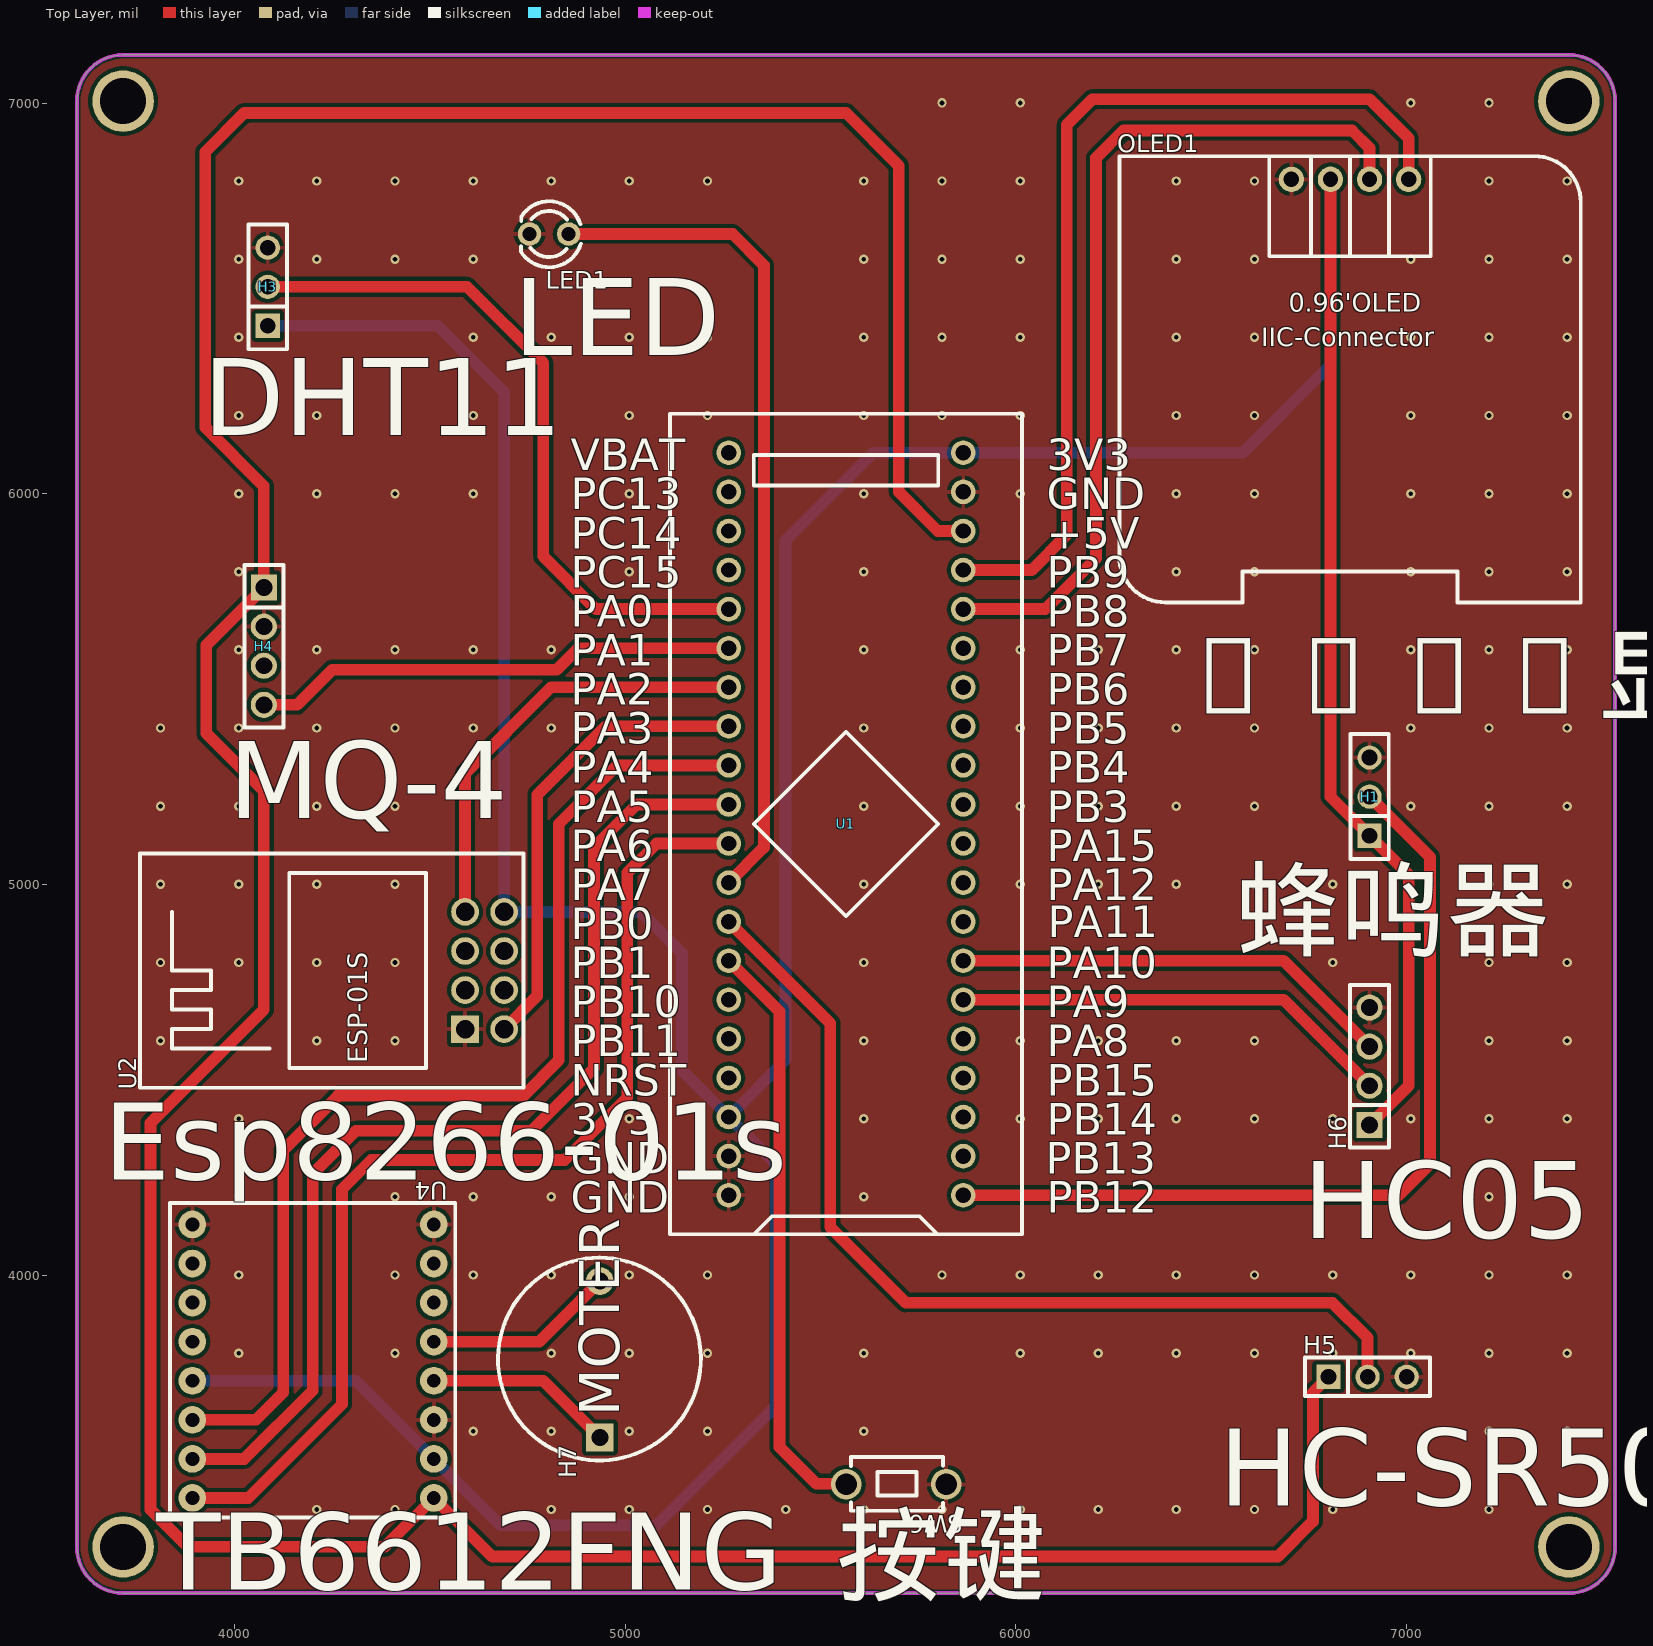
[diagram p0: Top Layer view]
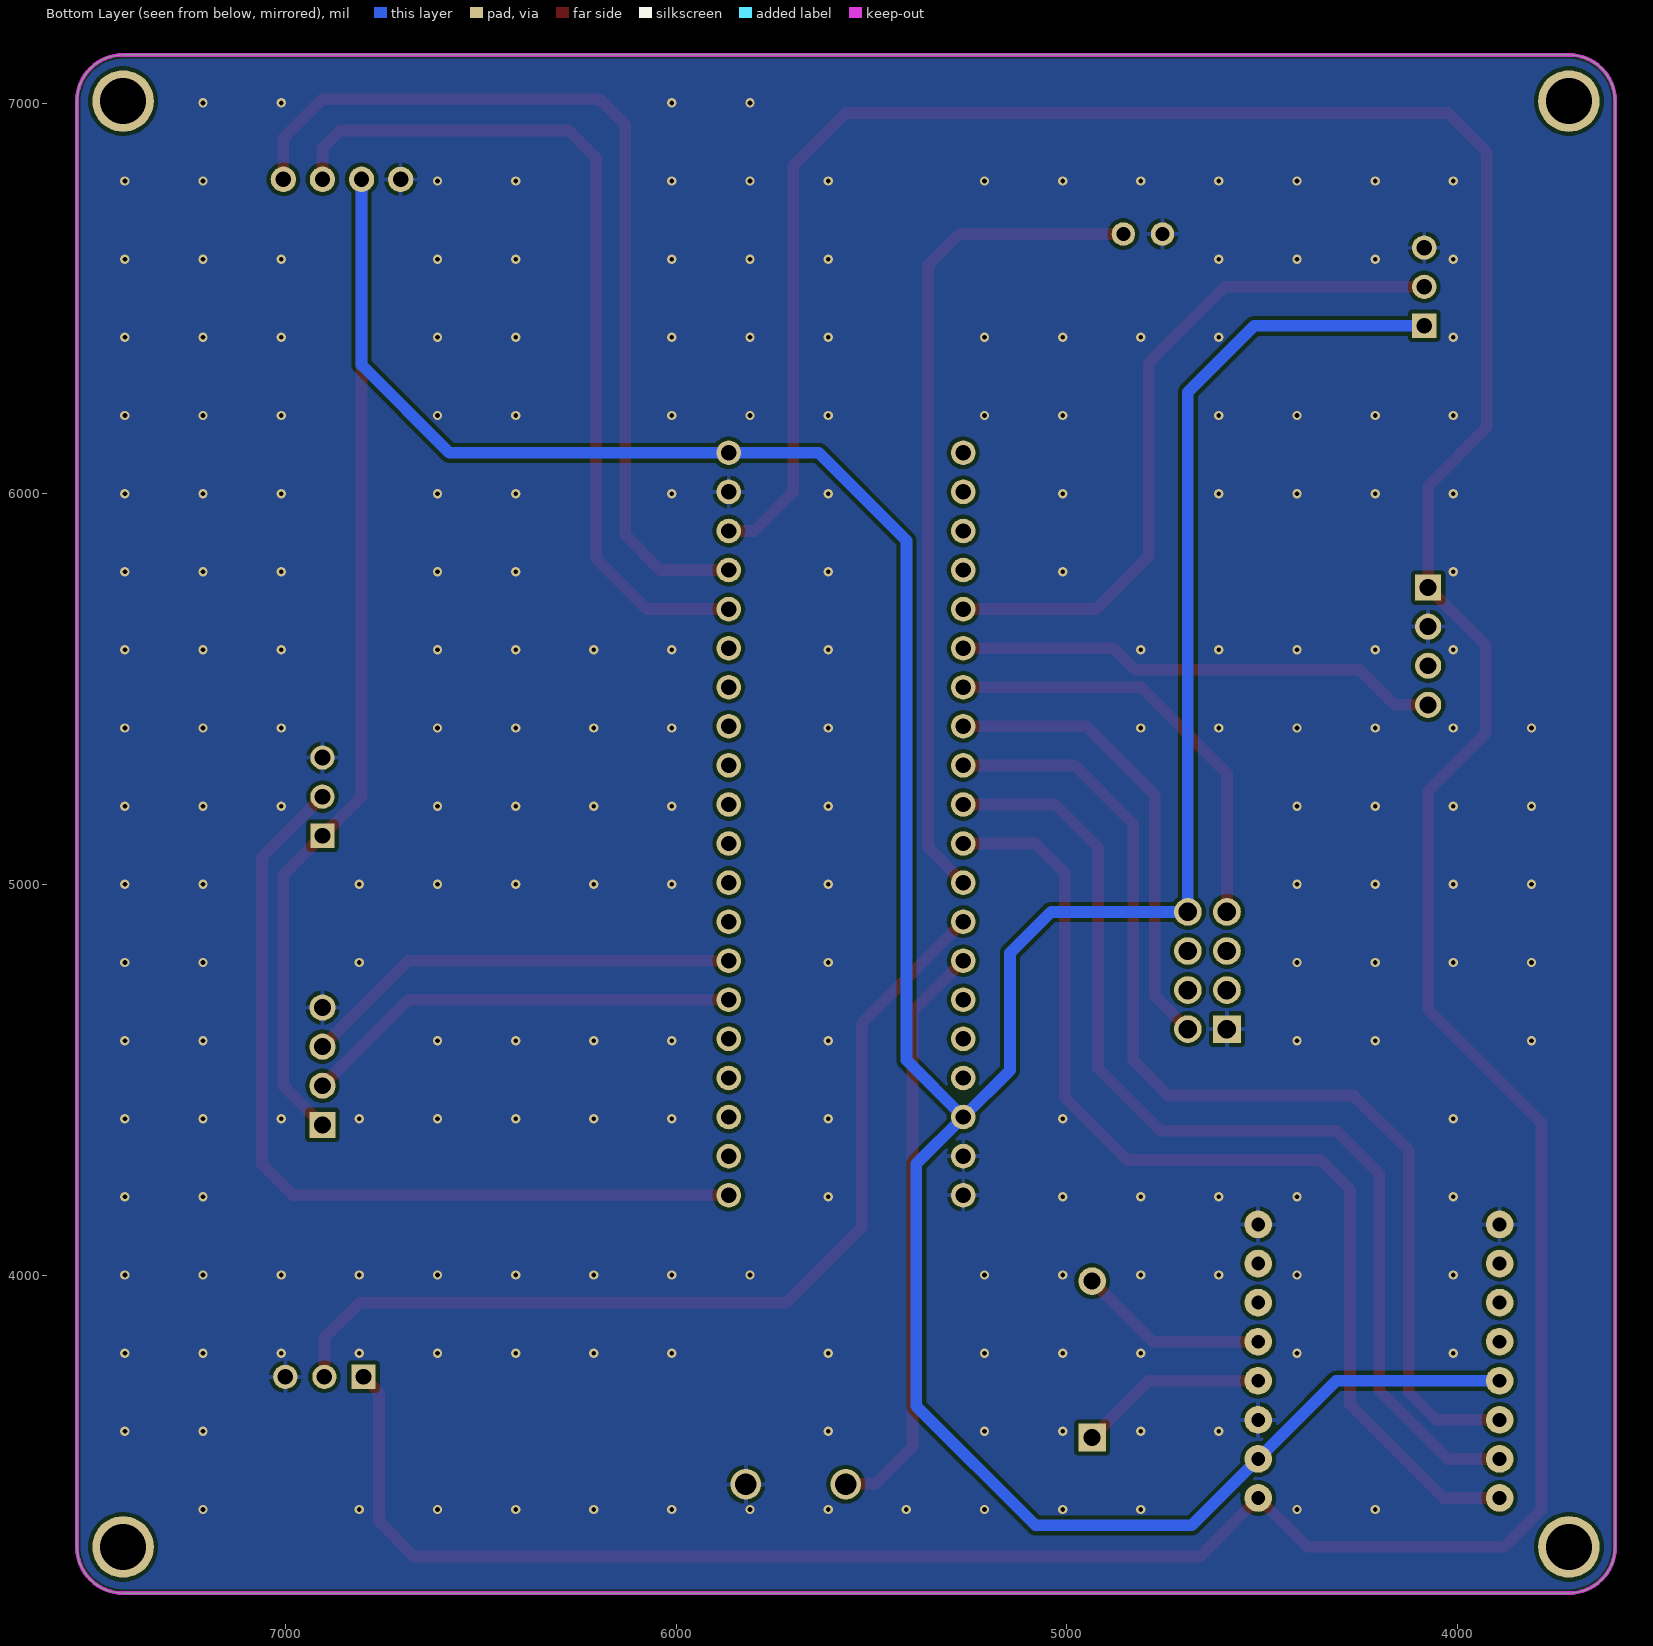
[diagram p1: Bottom Layer view, seen from below]
# Altium PCB MISC50942.pcbdoc
Units mil, origin at the board's own origin, x right, y up, seen from the top; angles counter-clockwise.
Board outline 3937.01 x 3937.01 mil, 2 copper layers (Top Layer, Bottom Layer), stack 62.206 mil thick; 12 components, 39 nets, 95 pads, 215 vias.

## Layer stack, top to bottom
Top Solder Mask Layer: solder mask 0.394, Dk 3.3
Top Layer: signal copper 1.379
Dielectric1: surface 59.449, FR4, Dk 4.5
Bottom Layer: signal copper 1.378
Bottom Solder Mask Layer: solder mask 0.394, Dk 3.3

## Board outline
3714.61,7123.5 ccw(c3714.61,7005.39) 3596.5,7005.39 3596.5,3304.61 ccw(c3714.61,3304.61) 3714.61,3186.5 7415.39,3186.5 ccw(c7415.39,3304.61) 7533.5,3304.61 7533.5,7005.39 ccw(c7415.39,7005.39) 7415.39,7123.5 3714.61,7123.5

## Design rules (kind name [scope] priority, off if disabled: settings)
BoardOutlineClearance copperThickness2oz_1 [All] p2 off: genericclearance=7.99 ignorepadtopadclearanceinfootprint=FALSE except(0: Arc-SplitContinuation Track-SplitContinuation SMDPad-SplitContinuation THPad-SplitContinuation Via-SplitContinuation Fill-SplitContinuation Region-SplitContinuation Poly-SplitContinuation Text-SplitContinuation Hole-SplitContinuation; 5.98: Arc-CutoutEdge Track-CutoutEdge SMDPad-CutoutEdge THPad-CutoutEdge Via-CutoutEdge Text-CutoutEdge; 6.9: Hole-OutlineEdge Hole-CutoutEdge; 10: Poly-OutlineEdge Poly-CutoutEdge; 11.81: Arc-OutlineEdge Track-OutlineEdge SMDPad-OutlineEdge THPad-OutlineEdge Via-OutlineEdge Fill-OutlineEdge Region-OutlineEdge Text-OutlineEdge Fill-CutoutEdge Region-CutoutEdge)
BoardOutlineClearance Plane_innerPlane_1 [All] p4 off: genericclearance=4.02 ignorepadtopadclearanceinfootprint=FALSE except(0: Arc-SplitContinuation Track-SplitContinuation SMDPad-SplitContinuation THPad-SplitContinuation Via-SplitContinuation Fill-SplitContinuation Region-SplitContinuation Poly-SplitContinuation Text-SplitContinuation Hole-SplitContinuation; 5.98: Arc-CutoutEdge Track-CutoutEdge SMDPad-CutoutEdge THPad-CutoutEdge Via-CutoutEdge Text-CutoutEdge; 6.9: Hole-OutlineEdge Hole-CutoutEdge; 10: Poly-OutlineEdge Poly-CutoutEdge; 11.81: Arc-OutlineEdge Track-OutlineEdge SMDPad-OutlineEdge THPad-OutlineEdge Via-OutlineEdge Fill-OutlineEdge Region-OutlineEdge Text-OutlineEdge Fill-CutoutEdge Region-CutoutEdge)
BoardOutlineClearance Copper_copperRegion_1 [All] p6 off: genericclearance=4.02 ignorepadtopadclearanceinfootprint=FALSE except(0: Arc-SplitContinuation Track-SplitContinuation SMDPad-SplitContinuation THPad-SplitContinuation Via-SplitContinuation Fill-SplitContinuation Region-SplitContinuation Poly-SplitContinuation Text-SplitContinuation Hole-SplitContinuation; 5.98: Arc-CutoutEdge Track-CutoutEdge SMDPad-CutoutEdge THPad-CutoutEdge Via-CutoutEdge Text-CutoutEdge; 6.9: Hole-OutlineEdge Hole-CutoutEdge; 10: Poly-OutlineEdge Poly-CutoutEdge; 11.81: Arc-OutlineEdge Track-OutlineEdge SMDPad-OutlineEdge THPad-OutlineEdge Via-OutlineEdge Fill-OutlineEdge Region-OutlineEdge Text-OutlineEdge Fill-CutoutEdge Region-CutoutEdge)
BoardOutlineClearance Copper_copperRegion_copperThickness1oz_1 [All] p8 off: genericclearance=4.02 ignorepadtopadclearanceinfootprint=FALSE except(0: Arc-SplitContinuation Track-SplitContinuation SMDPad-SplitContinuation THPad-SplitContinuation Via-SplitContinuation Fill-SplitContinuation Region-SplitContinuation Poly-SplitContinuation Text-SplitContinuation Hole-SplitContinuation; 5.98: Arc-CutoutEdge Track-CutoutEdge SMDPad-CutoutEdge THPad-CutoutEdge Via-CutoutEdge Text-CutoutEdge; 6.9: Hole-OutlineEdge Hole-CutoutEdge; 10: Poly-OutlineEdge Poly-CutoutEdge; 11.81: Arc-OutlineEdge Track-OutlineEdge SMDPad-OutlineEdge THPad-OutlineEdge Via-OutlineEdge Fill-OutlineEdge Region-OutlineEdge Text-OutlineEdge Fill-CutoutEdge Region-CutoutEdge)
BoardOutlineClearance Copper_copperRegion_Copper_copperRegion_1 [All] p10 off: genericclearance=4.02 ignorepadtopadclearanceinfootprint=FALSE except(0: Arc-SplitContinuation Track-SplitContinuation SMDPad-SplitContinuation THPad-SplitContinuation Via-SplitContinuation Fill-SplitContinuation Region-SplitContinuation Poly-SplitContinuation Text-SplitContinuation Hole-SplitContinuation; 5.98: Arc-CutoutEdge Track-CutoutEdge SMDPad-CutoutEdge THPad-CutoutEdge Via-CutoutEdge Text-CutoutEdge; 6.9: Hole-OutlineEdge Hole-CutoutEdge; 10: Poly-OutlineEdge Poly-CutoutEdge; 11.81: Arc-OutlineEdge Track-OutlineEdge SMDPad-OutlineEdge THPad-OutlineEdge Via-OutlineEdge Fill-OutlineEdge Region-OutlineEdge Text-OutlineEdge Fill-CutoutEdge Region-CutoutEdge)
BoardOutlineClearance copperThickness1oz_1 [All] p12: genericclearance=4.02 ignorepadtopadclearanceinfootprint=FALSE except(0: Arc-SplitContinuation Track-SplitContinuation SMDPad-SplitContinuation THPad-SplitContinuation Via-SplitContinuation Fill-SplitContinuation Region-SplitContinuation Poly-SplitContinuation Text-SplitContinuation Hole-SplitContinuation; 5.98: Arc-CutoutEdge Track-CutoutEdge SMDPad-CutoutEdge THPad-CutoutEdge Via-CutoutEdge Text-CutoutEdge; 6.9: Hole-OutlineEdge Hole-CutoutEdge; 10: Poly-OutlineEdge Poly-CutoutEdge; 11.81: Arc-OutlineEdge Track-OutlineEdge SMDPad-OutlineEdge THPad-OutlineEdge Via-OutlineEdge Fill-OutlineEdge Region-OutlineEdge Text-OutlineEdge Fill-CutoutEdge Region-CutoutEdge)
Clearance copperThickness2oz [All] p1 off: gap=7.99 ignorepadtopadclearanceinfootprint=FALSE except(5.98: SMDPad-Track SMDPad-SMDPad THPad-Track SMDPad-THPad THPad-THPad Track-Via SMDPad-Via THPad-Via Via-Via Fill-SMDPad Region-SMDPad Fill-THPad Region-THPad Fill-Via Region-Via Fill-Fill Fill-Region Region-Region Arc-Track Arc-SMDPad Arc-THPad Arc-Via Fill-Arc Region-Arc Arc-Arc Text-Track SMDPad-Text Text-THPad Text-Via Fill-Text Region-Text Arc-Text Text-Text; 6.9: Hole-Track Hole-SMDPad Hole-THPad Hole-Via Fill-Hole Region-Hole Hole-Arc Hole-Text; 10: Poly-Track Poly-SMDPad Poly-THPad Poly-Via Poly-Fill Poly-Region Poly-Poly Poly-Arc Poly-Text Poly-Hole; 11.81: Fill-Track Region-Track)
Clearance Plane_innerPlane [All] p3 off: gap=4.02 ignorepadtopadclearanceinfootprint=FALSE except(5.98: SMDPad-Track SMDPad-SMDPad THPad-Track SMDPad-THPad THPad-THPad Track-Via SMDPad-Via THPad-Via Via-Via Fill-SMDPad Region-SMDPad Fill-THPad Region-THPad Fill-Via Region-Via Fill-Fill Fill-Region Region-Region Arc-Track Arc-SMDPad Arc-THPad Arc-Via Fill-Arc Region-Arc Arc-Arc Text-Track SMDPad-Text Text-THPad Text-Via Fill-Text Region-Text Arc-Text Text-Text; 6.9: Hole-Track Hole-SMDPad Hole-THPad Hole-Via Fill-Hole Region-Hole Hole-Arc Hole-Text; 10: Poly-Track Poly-SMDPad Poly-THPad Poly-Via Poly-Fill Poly-Region Poly-Poly Poly-Arc Poly-Text Poly-Hole; 11.81: Fill-Track Region-Track)
Clearance Copper_copperRegion [All] p5 off: gap=4.02 ignorepadtopadclearanceinfootprint=FALSE except(5.98: SMDPad-Track SMDPad-SMDPad THPad-Track SMDPad-THPad THPad-THPad Track-Via SMDPad-Via THPad-Via Via-Via Fill-SMDPad Region-SMDPad Fill-THPad Region-THPad Fill-Via Region-Via Fill-Fill Fill-Region Region-Region Arc-Track Arc-SMDPad Arc-THPad Arc-Via Fill-Arc Region-Arc Arc-Arc Text-Track SMDPad-Text Text-THPad Text-Via Fill-Text Region-Text Arc-Text Text-Text; 6.9: Hole-Track Hole-SMDPad Hole-THPad Hole-Via Fill-Hole Region-Hole Hole-Arc Hole-Text; 10: Poly-Track Poly-SMDPad Poly-THPad Poly-Via Poly-Fill Poly-Region Poly-Poly Poly-Arc Poly-Text Poly-Hole; 11.81: Fill-Track Region-Track)
Clearance Copper_copperRegion_copperThickness1oz [All] p7 off: gap=4.02 ignorepadtopadclearanceinfootprint=FALSE except(5.98: SMDPad-Track SMDPad-SMDPad THPad-Track SMDPad-THPad THPad-THPad Track-Via SMDPad-Via THPad-Via Via-Via Fill-SMDPad Region-SMDPad Fill-THPad Region-THPad Fill-Via Region-Via Fill-Fill Fill-Region Region-Region Arc-Track Arc-SMDPad Arc-THPad Arc-Via Fill-Arc Region-Arc Arc-Arc Text-Track SMDPad-Text Text-THPad Text-Via Fill-Text Region-Text Arc-Text Text-Text; 6.9: Hole-Track Hole-SMDPad Hole-THPad Hole-Via Fill-Hole Region-Hole Hole-Arc Hole-Text; 10: Poly-Track Poly-SMDPad Poly-THPad Poly-Via Poly-Fill Poly-Region Poly-Poly Poly-Arc Poly-Text Poly-Hole; 11.81: Fill-Track Region-Track)
Clearance Copper_copperRegion_Copper_copperRegion [All] p9 off: gap=4.02 ignorepadtopadclearanceinfootprint=FALSE except(5.98: SMDPad-Track SMDPad-SMDPad THPad-Track SMDPad-THPad THPad-THPad Track-Via SMDPad-Via THPad-Via Via-Via Fill-SMDPad Region-SMDPad Fill-THPad Region-THPad Fill-Via Region-Via Fill-Fill Fill-Region Region-Region Arc-Track Arc-SMDPad Arc-THPad Arc-Via Fill-Arc Region-Arc Arc-Arc Text-Track SMDPad-Text Text-THPad Text-Via Fill-Text Region-Text Arc-Text Text-Text; 6.9: Hole-Track Hole-SMDPad Hole-THPad Hole-Via Fill-Hole Region-Hole Hole-Arc Hole-Text; 10: Poly-Track Poly-SMDPad Poly-THPad Poly-Via Poly-Fill Poly-Region Poly-Poly Poly-Arc Poly-Text Poly-Hole; 11.81: Fill-Track Region-Track)
Clearance copperThickness1oz [All] p11: gap=4.02 ignorepadtopadclearanceinfootprint=FALSE except(5.98: SMDPad-Track SMDPad-SMDPad THPad-Track SMDPad-THPad THPad-THPad Track-Via SMDPad-Via THPad-Via Via-Via Fill-SMDPad Region-SMDPad Fill-THPad Region-THPad Fill-Via Region-Via Fill-Fill Fill-Region Region-Region Arc-Track Arc-SMDPad Arc-THPad Arc-Via Fill-Arc Region-Arc Arc-Arc Text-Track SMDPad-Text Text-THPad Text-Via Fill-Text Region-Text Arc-Text Text-Text; 6.9: Hole-Track Hole-SMDPad Hole-THPad Hole-Via Fill-Hole Region-Hole Hole-Arc Hole-Text; 10: Poly-Track Poly-SMDPad Poly-THPad Poly-Via Poly-Fill Poly-Region Poly-Poly Poly-Arc Poly-Text Poly-Hole; 11.81: Fill-Track Region-Track)
DiffPairsRouting differentialPair [All] p1: maxlimit=6 minlimit=6 mostfreqgap=6 toplayer_minwidth=5 toplayer_prefwidth=10 toplayer_maxwidth=100 toplayer_mingap=6 toplayer_prefgap=6 toplayer_maxgap=6 bottomlayer_minwidth=5 bottomlayer_prefwidth=10 bottomlayer_maxwidth=100 bottomlayer_mingap=6 bottomlayer_prefgap=6 bottomlayer_maxgap=6 maxuncoupledlength=10
HoleToHoleClearance otherClearance [All] p1: gap=11.81 allowstackedmicrovias=TRUE
Length netLength [All] p1: minlimit=0 maxlimit=0
PasteMaskExpansion pasteMaskExpansion [All] p1: expansion=0
PlaneConnect innerPlane [All] p1: planeconnectstyle=Relief reliefexpansion=20 reliefentries=4 reliefconductorwidth=10 reliefairgap=10
PolygonConnect copperRegion_copperThickness1oz [All] p1 off: connectstyle=Relief reliefconductorwidth=10 reliefentries=4 polygonreliefangle="90 Angle" airgapwidth=10 via.connectstyle=Relief via.reliefconductorwidth=10 via.reliefentries=4 via.polygonreliefangle="90 Angle" via.airgapwidth=10
PolygonConnect copperRegion_Copper_copperRegion [All] p2 off: connectstyle=Relief reliefconductorwidth=10 reliefentries=4 polygonreliefangle="90 Angle" airgapwidth=10 via.connectstyle=Relief via.reliefconductorwidth=10 via.reliefentries=4 via.polygonreliefangle="90 Angle" via.airgapwidth=10
PolygonConnect copperRegion [All] p3: connectstyle=Relief reliefconductorwidth=10 reliefentries=4 polygonreliefangle="90 Angle" airgapwidth=10 via.connectstyle=Relief via.reliefconductorwidth=10 via.reliefentries=4 via.polygonreliefangle="90 Angle" via.airgapwidth=10
RoutingVias viaSize [All] p1: holewidth=12.01 width=24.02 viastyle="Through Hole" minholewidth=11.81 minwidth=19.68 maxholewidth=248.03 maxwidth=393.7
SolderMaskExpansion solderMaskExpansion [IsVia] p1: expansion=-1000 istentingtop=TRUE
SolderMaskExpansion solderMaskExpansion [All] p2: expansion=2 istentingtop=FALSE
Width copperThickness2oz_2 [All] p1 off: maxlimit=100 minlimit=8 preferedwidth=10
Width copperThickness1oz_2 [All] p2: maxlimit=100 minlimit=5 preferedwidth=10

## Components (designator, comment, footprint, x,y, rotation, side; value= is the part's Value field where it differs from the comment)
H1 "" HDR-TH_3P-P2.54-V-F 6905,5225 r90 top
H3 "" HDR-TH_3P-P2.54-V-F 4085,6530 r90 top
H4 "" HDR-TH_4P-P2.54-V-F 4075,5610 r270 top
H5 "" HDR-TH_3P-P2.54-V-F 6900,3740 r0 top
H6 "" HDR-TH_4P-P2.54-V-F 6905,4535 r90 top
H7 "" HDR-TH_2P-P2.54-V-M-1 4935,3585 r90 top
LED1 "" LED_TH-3mm 4805,6665 r180 top
OLED1 "" 0.96OLED_4P 6855,6805 r0 top
SW6 "" Key_TH_3.5x6x4.3 5700,3465 r180 top
U1 "STM32F103C8T6-Card" CONN-TH_L53.3-W22.9_STM32F103C8T6-CARD 5565,5155 r90 top
U2 "ESP-01S" WIFIM-TH_ESP-01S 4640,4780 r90 top
U4 "" tb6612 4510,3430 r180 top

## Footprints (in the part's own frame and the unit in brackets; to place one, negate y for a bottom-side part, rotate by r counter-clockwise, add the part's x,y. Pads: shape width x height; smd on the part's side, far side on the other; paste and mask are expansions set on the pad)
0.96OLED_4P [mm]
  round 1.65 hole 1 copper offset 0,0: 1(-3.81,-0.001) 2(-1.27,0.002) 3(1.27,0.002) 4(3.81,0.002)
  silkscreen extent -15,-27.5 15,1.5
CONN-TH_L53.3-W22.9_STM32F103C8T6-CARD [mm]
  round 1.6 hole 1: 1(-24.13,-7.62) 2(-21.59,-7.62) 3(-19.05,-7.62) 4(-16.51,-7.62) 5(-13.97,-7.62) 6(-11.43,-7.62) 7(-8.89,-7.62) 8(-6.35,-7.62) 9(-3.81,-7.62) 10(-1.27,-7.62) 11(1.27,-7.62) 12(3.81,-7.62) 13(6.35,-7.62) 14(8.89,-7.62) 15(11.43,-7.62) 16(13.97,-7.62) 17(16.51,-7.62) 18(19.05,-7.62) 19(21.59,-7.62) 20(24.13,-7.62) 21(24.13,7.62) 22(21.59,7.62) 23(19.05,7.62) 24(16.51,7.62) 25(13.97,7.62) 26(11.43,7.62) 27(8.89,7.62) 28(6.35,7.62) 29(3.81,7.62) 30(1.27,7.62) 31(-1.27,7.62) 32(-3.81,7.62) 33(-6.35,7.62) 34(-8.89,7.62) 35(-11.43,7.62) 36(-13.97,7.62) 37(-16.51,7.62) 38(-19.05,7.62) 39(-21.59,7.62) 40(-24.13,7.62)
  silkscreen extent -26.67,-11.43 26.67,11.43
HDR-TH_2P-P2.54-V-M-1 [mm]
  rect 1.8x1.8 hole 1.1: 1(0,0)
  round 1.8 hole 1.1: 2(10.16,0)
  silkscreen extent -1.49,-6.56 11.69,6.62
HDR-TH_3P-P2.54-V-F [mil]
  rect 62x62 hole 40.16: 1(-100,0)
  round 62 hole 40.16: 2(0,0) 3(100,0)
  silkscreen extent -160,-49 160,49
HDR-TH_4P-P2.54-V-F [mm]
  rect 1.7x1.7 hole 1.1: 1(-3.81,0)
  round 1.7 hole 1.1: 2(-1.27,0) 3(1.27,0) 4(3.81,0)
  silkscreen extent -5.29,-1.27 5.29,1.27
Key_TH_3.5x6x4.3 [mil]
  round 78.7 hole 55.1 paste+0 mask+2: A(-121.44,0) B(134.46,0)
  silkscreen extent -114,-70 123,68
LED_TH-3mm [mil]
  round 60 hole 36 paste+0 mask+2: 1(-50,0) 2(50,0)
  silkscreen extent -81,-84 72,85
tb6612 [mm]
  round 1.8 hole 0.9: 1(0,0) 2(0,-2.54) 3(0,-5.08) 4(0,-7.62) 5(0,-10.16) 6(0,-12.7) 7(0,-15.24) 8(0,-17.78) 9(15.697,-17.78) 10(15.697,-15.24) 11(15.697,-12.7) 12(15.697,-10.16) 13(15.697,-7.62) 14(15.697,-5.08) 15(15.697,-2.54) 16(15.697,0)
  silkscreen extent -1.4,-19.18 17.15,1.27
WIFIM-TH_ESP-01S [mm]
  rect 1.8x1.8 hole 1.2: 1(-3.81,1.27)
  round 1.8 hole 1.2: 2(-1.27,1.27) 3(1.27,1.27) 4(3.81,1.27) 5(3.81,-1.27) 6(1.27,-1.27) 7(-1.27,-1.27) 8(-3.81,-1.27)
  silkscreen extent -7.62,-2.54 7.62,22.4

## Free pads (board coordinates)
  round 157.48 hole 118.11: 1(3714.61,7005.39) 1(3714.61,3304.61) 1(7415.39,7005.39) 1(7415.39,3304.61)

## Via types
v1: diameter 24.02, hole 12, Top Layer to Bottom Layer, 215 vias

## Nets (pads, with @x,y where several pads share a name; then routed paths per layer and width w, separated by ;. In a path a pad name is that pad's centre, name@x,y a point inside that pad or via, vN(x,y) a via of type N, cw(c..) or ccw(c..) an arc to the next point about the centre after c; other vN are vias at no path point)
$1N17162: H7.1 U4.4 | length 485.1
  Top Layer w30: U4.4 4790,3730 H7.1
$1N17163: H7.2 U4.5 | length 489.2
  Top Layer w30: U4.5 4780,3830 H7.2
+5V: H4.1 H5.1 U1.18 U4.1 | length 10245
  Top Layer w30: U1.18 5800,5905 5700,6005 5700,6840 5565,6975 4025,6975 3925,6875 3925,6170 4075,6020 H4.1 3927.93,5612.93 3927.93,5387.07 4075,5240 4075,4680 3785,4390 3785,3400 3880,3305 4385,3305 U4.1 4660,3280 6670,3280 6760,3370 6760,3700 H5.1
GND: H1.3 H3.3 H4.2 H5.3 H6.4 LED1.2 OLED1.1 SW6.A U1.19 U1.39 U1.40 U2.1 U4.3 U4.8 U4.9
  other v1: 4210.6,3400.6 4410.6,3400.6 4810.6,3400.6 5010.6,3400.6 5210.6,3400.6 5410.6,3400.6 5610.6,3400.6 5810.6,3400.6 6010.6,3400.6 6210.6,3400.6 6410.6,3400.6 6610.6,3400.6 6810.6,3400.6 7210.6,3400.6 4610.6,3600.6 4810.6,3600.6 5010.6,3600.6 5210.6,3600.6 5610.6,3600.6 7210.6,3600.6 7410.6,3600.6 4010.6,3800.6 4410.6,3800.6 4810.6,3800.6 5010.6,3800.6 5210.6,3800.6 5610.6,3800.6 6010.6,3800.6 6210.6,3800.6 6410.6,3800.6 6610.6,3800.6 6810.6,3800.6 7010.6,3800.6 7210.6,3800.6 7410.6,3800.6 4010.6,4000.6 4410.6,4000.6 4610.6,4000.6 4810.6,4000.6 5010.6,4000.6 5210.6,4000.6 5810.6,4000.6 6010.6,4000.6 6210.6,4000.6 6410.6,4000.6 6610.6,4000.6 6810.6,4000.6 7010.6,4000.6 7210.6,4000.6 7410.6,4000.6 4010.6,4200.6 4410.6,4200.6 4610.6,4200.6 4810.6,4200.6 5010.6,4200.6 5610.6,4200.6 7210.6,4200.6 7410.6,4200.6 4010.6,4400.6 5010.6,4400.6 5610.6,4400.6 6010.6,4400.6 6210.6,4400.6 6410.6,4400.6 6610.6,4400.6 6810.6,4400.6 7010.6,4400.6 7210.6,4400.6 7410.6,4400.6 3810.6,4600.6 4210.6,4600.6 4410.6,4600.6 5610.6,4600.6 6010.6,4600.6 6210.6,4600.6 6410.6,4600.6 6610.6,4600.6 7210.6,4600.6 7410.6,4600.6 3810.6,4800.6 4010.6,4800.6 4210.6,4800.6 4410.6,4800.6 5610.6,4800.6 6810.6,4800.6 7210.6,4800.6 7410.6,4800.6 3810.6,5000.6 4010.6,5000.6 4210.6,5000.6 4410.6,5000.6 5610.6,5000.6 6010.6,5000.6 6210.6,5000.6 6410.6,5000.6 6610.6,5000.6 6810.6,5000.6 7210.6,5000.6 7410.6,5000.6 3810.6,5200.6 4010.6,5200.6 4210.6,5200.6 4410.6,5200.6 5610.6,5200.6 6010.6,5200.6 6210.6,5200.6 6410.6,5200.6 6610.6,5200.6 7010.6,5200.6 7210.6,5200.6 7410.6,5200.6 3810.6,5400.6 4010.6,5400.6 4210.6,5400.6 4410.6,5400.6 4610.6,5400.6 4810.6,5400.6 5610.6,5400.6 6010.6,5400.6 6210.6,5400.6 6410.6,5400.6 6610.6,5400.6 7010.6,5400.6 7210.6,5400.6 7410.6,5400.6 4010.6,5600.6 4210.6,5600.6 4410.6,5600.6 4610.6,5600.6 4810.6,5600.6 5610.6,5600.6 6010.6,5600.6 6210.6,5600.6 6410.6,5600.6 6610.6,5600.6 7010.6,5600.6 7210.6,5600.6 7410.6,5600.6 4010.6,5800.6 5010.6,5800.6 5610.6,5800.6 6410.6,5800.6 6610.6,5800.6 7010.6,5800.6 7210.6,5800.6 7410.6,5800.6 4010.6,6000.6 4210.6,6000.6 4410.6,6000.6 4610.6,6000.6 5010.6,6000.6 5610.6,6000.6 6010.6,6000.6 6410.6,6000.6 6610.6,6000.6 7010.6,6000.6 7210.6,6000.6 7410.6,6000.6 4010.6,6200.6 4210.6,6200.6 4410.6,6200.6 4610.6,6200.6 5010.6,6200.6 5210.6,6200.6 5610.6,6200.6 5810.6,6200.6 6010.6,6200.6 6410.6,6200.6 6610.6,6200.6 7010.6,6200.6 7210.6,6200.6 7410.6,6200.6 4010.6,6400.6 4610.6,6400.6 4810.6,6400.6 5010.6,6400.6 5210.6,6400.6 5610.6,6400.6 5810.6,6400.6 6010.6,6400.6 6410.6,6400.6 6610.6,6400.6 7010.6,6400.6 7210.6,6400.6 7410.6,6400.6 4010.6,6600.6 4210.6,6600.6 4410.6,6600.6 4610.6,6600.6 5610.6,6600.6 5810.6,6600.6 6010.6,6600.6 6410.6,6600.6 6610.6,6600.6 7010.6,6600.6 7210.6,6600.6 7410.6,6600.6 4010.6,6800.6 4210.6,6800.6 4410.6,6800.6 4610.6,6800.6 4810.6,6800.6 5010.6,6800.6 5210.6,6800.6 5610.6,6800.6 5810.6,6800.6 6010.6,6800.6 6410.6,6800.6 6610.6,6800.6 7210.6,6800.6 7410.6,6800.6 5810.6,7000.6 6010.6,7000.6 7010.6,7000.6 7210.6,7000.6
NRST: U1.37
PA0: H3.2 U1.25 | length 1811.7
  Top Layer w30: H3.2 4595,6530 4790,6335 4790,5840 4925,5705 U1.25
PA1: H4.4 U1.26 | length 1250.1
  Top Layer w30: H4.4 4160,5460 4250,5550 4825,5550 4880,5605 U1.26
PA2: U1.27 U2.4 | length 1121.1
  Top Layer w30: U2.4 4590,5285 4810,5505 U1.27
PA3: U1.28 U2.8 | length 1197.7
  Top Layer w30: U2.8 4775,4715 4775,5230 4950,5405 U1.28
PA4: U1.29 U4.14 | length 2784.4
  Top Layer w30: U4.14 4055,3630 4125,3700 4125,4320 4265,4460 4740,4460 4830,4550 4830,5155 4980,5305 U1.29
PA5: U1.30 U4.15 | length 2722.9
  Top Layer w30: U4.15 4025,3530 4200,3705 4200,4260 4310,4370 4760,4370 4920,4530 4920,5095 5030,5205 U1.30
PA6: U1.31 U4.16 | length 2725.8
  Top Layer w30: U4.16 4035,3430 4275,3670 4275,4220 4350,4295 4845,4295 5005,4455 5005,5030 5080,5105 U1.31
PA7: LED1.1 U1.32 | length 2150.4
  Top Layer w30: LED1.1 5275,6665 5355,6585 5355,5095 U1.32
PA8: U1.5
PA9: H6.2 U1.6 | length 1131.1
  Top Layer w30: U1.6 6685,4705 H6.2
PA10: H6.3 U1.7 | length 1131.1
  Top Layer w30: U1.7 6685,4805 H6.3
PA11: U1.8
PA12: U1.9
PA15: U1.10
PB0: H5.2 U1.33 | length 2481.8
  Top Layer w30: U1.33 5525,4645 5525,4123.27 5718.27,3930 6810,3930 6900,3840 H5.2
PB1: SW6.B U1.34 | length 1504.7
  Top Layer w30: U1.34 5395,4675 5395,3560 5488.58,3466.42 SW6.B@5562.05,3466.42
PB3: U1.11
PB4: U1.12
PB5: U1.13
PB6: U1.14
PB7: U1.15
PB8: OLED1.3 U1.16 | length 2246.4
  Top Layer w30: U1.16 6075,5705 6205,5835 6205,6860 6275,6930 6860,6930 6905,6885 OLED1.3@6905,6805.05
PB9: OLED1.4 U1.17 | length 2400.6
  Top Layer w30: U1.17 6040,5805 6130,5895 6130,6945 6195,7010 6905,7010 7005,6910 OLED1.4@7005,6805.05
PB10: U1.35
PB11: U1.36
PB12: H1.2 U1.1 | length 2232.3
  Top Layer w30: U1.1 6980,4205 7060,4285 7060,5070 H1.2
PB13: U1.2
PB14: U1.3
PB15: U1.4
PC13: U1.22
PC14: U1.23
PC15: U1.24
VBAT: U1.21
VCC: H1.1 H3.1 H6.1 OLED1.2 U1.20 U1.38 U2.5 U4.2 U4.13 | length 11671.7
  Top Layer w30: OLED1.2@6805,6805.05 6805,5225 H1.1 7005,5025 7005,4485 H6.1
  Bottom Layer w30: U4.13 4310,3730 U4.2 4680,3360 5080,3360 5385,3665 5385,4285 U1.38 ; H3.1 4520,6430 4690,6260 U2.5 5040,4930 5145,4825 5145,4525 U1.38 ; OLED1.2@6805,6805.05 6805,6330 6580,6105 U1.20 5635,6105 5410,5880 5410,4550 U1.38
pads on no net: H4.3 U2.2 U2.3 U2.6 U2.7 U4.6 U4.7 U4.10 U4.11 U4.12

## Polygon pours and split planes (outlines as drawn)
GND on Bottom Layer (solid, remove dead copper, pour order 2): 3525,7245 3525,3080 7700,3080 7700,7245
GND on Top Layer (solid, remove dead copper, pour order 2): 3000,7415 3000,3000 7930,3000 7930,7415

## Keep-outs
Board Outline Layer:
  the board outline again, w10

## Silkscreen, mask and mechanical layers (free items; w line width, h text height)
Top Silkscreen Layer:
  text "LED" at 4715,6355 h196.85
  text "DHT11" at 3920,6150 h196.85
  text "VBAT" at 4860.95,6060 h80
  text "3V3" at 6079.16,6060 h80
  text "PC13" at 4860.95,5960 h80
  text "GND" at 6079.16,5960 h80
  text "PC14" at 4860.95,5860 h80
  text "+5V" at 6079.16,5860 h80
  text "PC15" at 4860.95,5760 h80
  text "PB9" at 6079.16,5760 h80
  text "PA0" at 4860.95,5660 h80
  text "PB8" at 6079.16,5660 h80
  text "PA1" at 4860.95,5560 h80
  text "PB7" at 6079.16,5560 h80
  text "PA2" at 4860.95,5460 h80
  text "PB6" at 6079.16,5460 h80
  text "Oled显示器" at 6408.66,5436.57 h196.85
  text "PA3" at 4860.95,5360 h80
  text "PB5" at 6079.16,5360 h80
  text "PA4" at 4860.95,5260 h80
  text "PB4" at 6079.16,5260 h80
  text "MQ-4" at 3985,5170 h196.85
  text "PA5" at 4860.95,5160 h80
  text "PB3" at 6079.16,5160 h80
  text "PA6" at 4860.95,5060 h80
  text "PA15" at 6079.16,5060 h80
  text "PA7" at 4860.95,4960 h80
  text "PA12" at 6079.16,4960 h80
  text "PA11" at 6080.95,4865 h80
  text "PB0" at 4860.95,4860 h80
  text "蜂鸣器" at 6560,4840 h196.85
  text "PB1" at 4860.95,4760 h80
  text "PA10" at 6079.16,4760 h80
  text "PB10" at 4860.95,4660 h80
  text "PA9" at 6079.16,4660 h80
  text "PB11" at 4860.95,4560 h80
  text "PA8" at 6079.16,4560 h80
  text "NRST" at 4860.95,4460 h80
  text "PB15" at 6079.16,4460 h80
  text "3V3" at 4860.95,4360 h80
  text "PB14" at 6079.16,4360 h80
  text "GND" at 4860.95,4260 h80
  text "PB13" at 6075.95,4260 h80
  text "Esp8266-01s" at 3665,4245 h196.85
  text "GND" at 4860.95,4160 h80
  text "PB12" at 6079.16,4160 h80
  text "HC05" at 6735,4095 h196.85
  text "HC-SR501" at 6520,3410 h196.85
  text "TB6612FNG" at 3800,3195 h196.85
  text "按键" at 5540,3190 h196.85